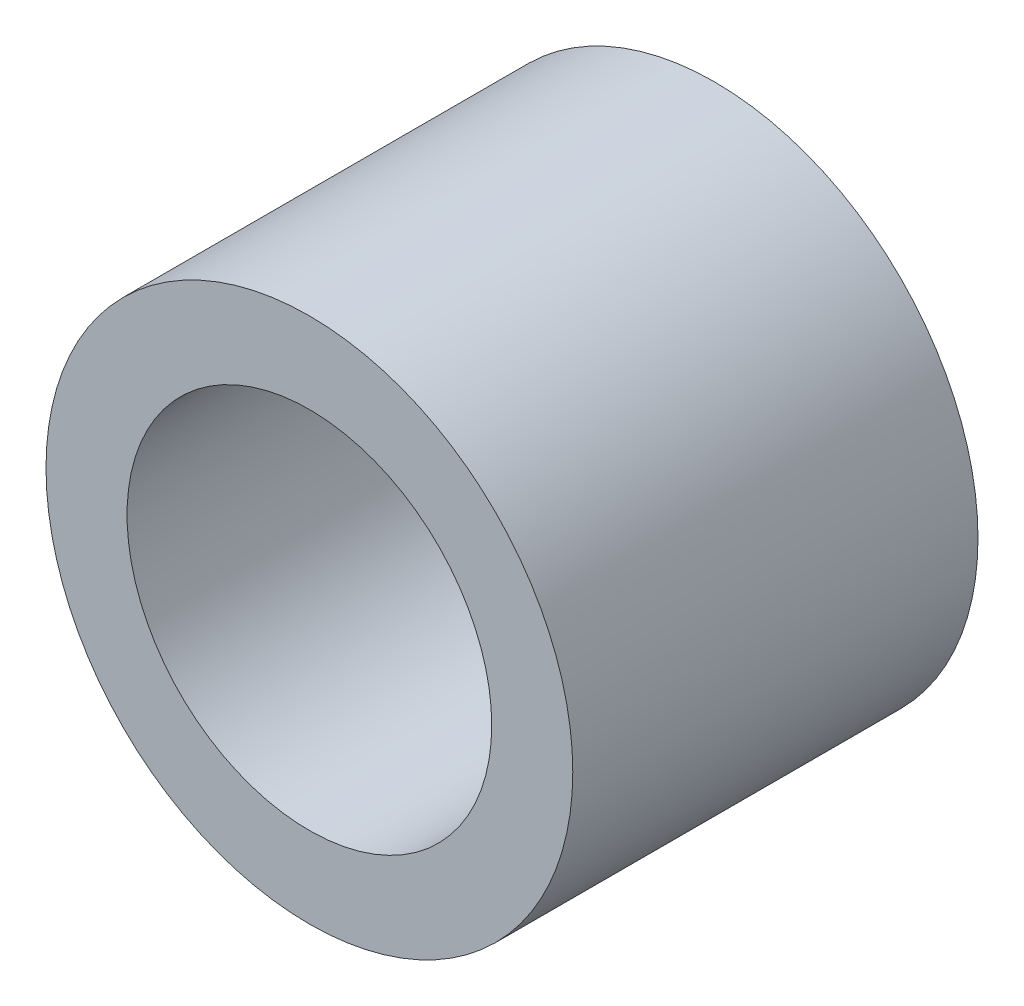
from build123d import *

# Parameters (mm, degrees)
SKETCH_1_R      = 32.5
SKETCH_1_R_2    = 22.5
EXTRUDE_1_DEPTH = 50


with BuildPart() as part:
    # 草图1 → 凸台-拉伸1 (new body)
    with BuildSketch(Plane.XY):
        Circle(SKETCH_1_R)
        Circle(SKETCH_1_R_2, mode=Mode.SUBTRACT)
    extrude(amount=EXTRUDE_1_DEPTH)


solid = part.part
